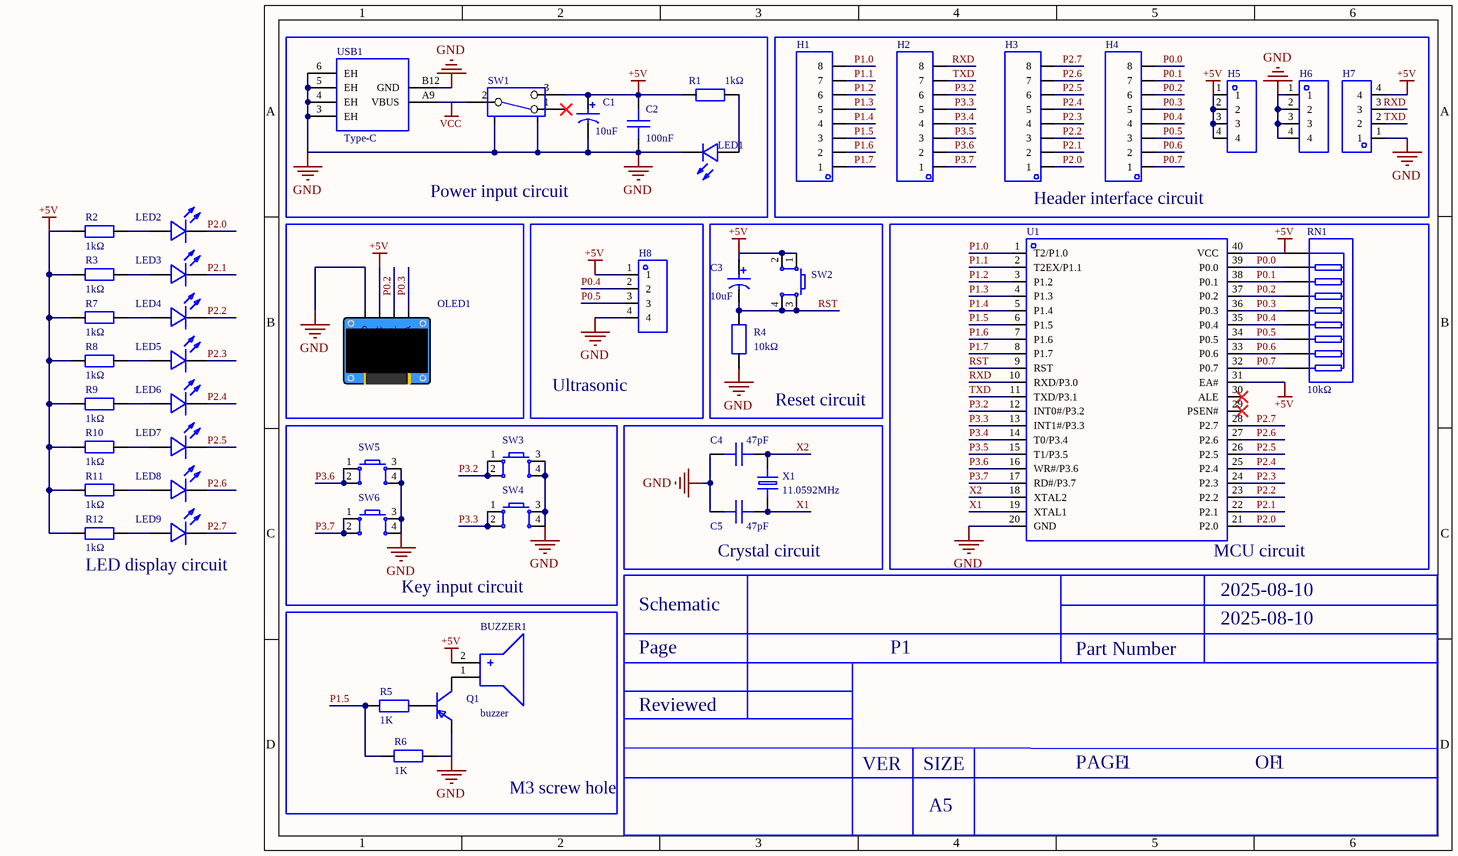
[diagram p0: MISC49889-2.schdoc]
# Altium project MISC49889-3.PrjPcb
1 sheet, 47 parts. Net scope: global (net labels, ports and power ports of the same name join across sheets).
Board file: MISC49889.pcbdoc

## Sheet MISC49889-2.schdoc
size 210 x 149 mm; Version: V1.0; @Project Name: MISC49889; @Page Count: 1; @Update Date: 2025-08-10; @Create Date: 2025-08-10; @Schematic Name: MISC49889; @Page No: 1; @Board Name: MISC49889; @Create Time: 18:24:45; @Update Time: 00:13:02

### Parts
BUZZER1  buzzer  [BUZ-TH_BD12.0-P6.00-D0.9-RD]
C1  10uF  [CAP-TH_BD5.0-P2.00-D0.8-FD]
C2  100nF  [CAP-TH_L8.5-W5.0-P5.00-D1.2]
C3  10uF  [CAP-TH_BD5.0-P2.00-D0.8-FD]
C4  47pF  [CAP-TH_L4.5-W3.0-P5.00-D1.2]
C5  47pF  [CAP-TH_L4.5-W3.0-P5.00-D1.2]
H1  (no value)  [HDR-TH_8P-P2.54-V-M]
H2  (no value)  [HDR-TH_8P-P2.54-V-M]
H3  (no value)  [HDR-TH_8P-P2.54-V-M]
H4  (no value)  [HDR-TH_8P-P2.54-V-M]
H5  (no value)  [HDR-TH_4P-P2.54-V-M]
H6  (no value)  [HDR-TH_4P-P2.54-V-M]
H7  (no value)  [HDR-TH_4P-P2.54-V-M]
H8  (no value)  [HDR-TH_4P-P2.54-V-F]
LED1  204-10SURD/S530-A3-L  [LED-TH_BD3.0-P2.54-FD]  (value not drawn)
LED2  204-10SYGD/S530-E3  [LED-TH_BD3.8-P2.54-FD]  (value not drawn)
LED3  204-10SYGD/S530-E3  [LED-TH_BD3.8-P2.54-FD]  (value not drawn)
LED4  204-10SYGD/S530-E3  [LED-TH_BD3.8-P2.54-FD]  (value not drawn)
LED5  204-10SYGD/S530-E3  [LED-TH_BD3.8-P2.54-FD]  (value not drawn)
LED6  204-10SYGD/S530-E3  [LED-TH_BD3.8-P2.54-FD]  (value not drawn)
LED7  204-10SYGD/S530-E3  [LED-TH_BD3.8-P2.54-FD]  (value not drawn)
LED8  204-10SYGD/S530-E3  [LED-TH_BD3.8-P2.54-FD]  (value not drawn)
LED9  204-10SYGD/S530-E3  [LED-TH_BD3.8-P2.54-FD]  (value not drawn)
OLED1  (no value)  [0.96OLED_4P]
Q1  (no value)  [S8550P_SOT]
R1  1kΩ  [RES-TH_BD2.5-L6.5-P10.50-D0.6]
R2  1kΩ  [RES-TH_BD2.5-L6.5-P10.50-D0.6]
R3  1kΩ  [RES-TH_BD2.5-L6.5-P10.50-D0.6]
R4  10kΩ  [RES-TH_BD2.4-L6.3-P10.30-D0.6]
R5  1K  [R0603]
R6  1K  [R0603]
R7  1kΩ  [RES-TH_BD2.5-L6.5-P10.50-D0.6]
R8  1kΩ  [RES-TH_BD2.5-L6.5-P10.50-D0.6]
R9  1kΩ  [RES-TH_BD2.5-L6.5-P10.50-D0.6]
R10  1kΩ  [RES-TH_BD2.5-L6.5-P10.50-D0.6]
R11  1kΩ  [RES-TH_BD2.5-L6.5-P10.50-D0.6]
R12  1kΩ  [RES-TH_BD2.5-L6.5-P10.50-D0.6]
RN1  10kΩ  [RES-ARRAY-TH_9P-P2.54-D1.0]
SW1  SS-12D02-VG4  [SW-TH_SS-12D02-VG4]  (value not drawn)
SW2  (no value)  [SW-TH_4P-L6.0-W6.0-P4.50-LS6.5]
SW3  (no value)  [SW-TH_4P-L6.0-W6.0-P4.50-LS6.5]
SW4  (no value)  [SW-TH_4P-L6.0-W6.0-P4.50-LS6.5]
SW5  (no value)  [SW-TH_4P-L6.0-W6.0-P4.50-LS6.5]
SW6  (no value)  [SW-TH_4P-L6.0-W6.0-P4.50-LS6.5]
U1  STC89C52RC-40I-PDIP40  [DIP-40_L52.0-W13.7-P2.54-LS15.2-BL]  (value not drawn)
USB1  Connector Type: Type-C  [USB-C-TH_TYPE-C-31-M-33]  (hidden comment: TYPE-C-31-M-33)
X1  11.0592MHz  [HC-49US_L11.5-W4.5-P4.88]

### Blocks framed on the sheet
Power input circuit: C1 C2 LED1 R1 SW1 USB1
Header interface circuit: H1-H7
Ultrasonic: H8
Reset circuit: C3 R4 SW2
MCU circuit: RN1 U1
Key input circuit: SW3-SW6
Crystal circuit: C4 C5 X1
M3 screw hole: BUZZER1 Q1 R5 R6

### Nets
+5V: BUZZER1.2(+) C1.1 C2.2 C3.1 H5.1 H5.2 H5.3 H5.4 H7.4 H8.1 OLED1.2(VCC) R1.1 R2.1 R3.1 R7.1 R8.1 R9.1 R10.1 R11.1 R12.1 RN1.1 SW1.3 SW2.1 SW2.2 U1.31(EA#) U1.40(VCC)
GND: C1.2 C2.1 C4.1 C5.1 H6.1 H6.2 H6.3 H6.4 H7.1 H8.4 LED1.2(K) OLED1.1(GND) Q1.2(E) R4.1 R6.2 SW1.4 SW1.5 SW3.3 SW3.4 SW4.3 SW4.4 SW5.3 SW5.4 SW6.3 SW6.4 U1.20(GND) USB1.3(EH) USB1.4(EH) USB1.5(EH) USB1.6(EH) USB1.B12(GND)
VCC: SW1.2 USB1.A9(VBUS)
P0.0: H4.8 RN1.2 U1.39(P0.0)
P0.1: H4.7 RN1.3 U1.38(P0.1)
P0.2: H4.6 OLED1.3(SCL) RN1.4 U1.37(P0.2)
P0.3: H4.5 OLED1.4(SDA) RN1.5 U1.36(P0.3)
P0.4: H4.4 H8.2 RN1.6 U1.35(P0.4)
P0.5: H4.3 H8.3 RN1.7 U1.34(P0.5)
P0.6: H4.2 RN1.8 U1.33(P0.6)
P0.7: H4.1 RN1.9 U1.32(P0.7)
P1.0: H1.8 U1.1(T2/P1.0)
P1.1: H1.7 U1.2(T2EX/P1.1)
P1.2: H1.6 U1.3(P1.2)
P1.3: H1.5 U1.4(P1.3)
P1.4: H1.4 U1.5(P1.4)
P1.5: H1.3 R5.1 R6.1 U1.6(P1.5)
P1.6: H1.2 U1.7(P1.6)
P1.7: H1.1 U1.8(P1.7)
P2.0: H3.1 LED2.2(K) U1.21(P2.0)
P2.1: H3.2 LED3.2(K) U1.22(P2.1)
P2.2: H3.3 LED4.2(K) U1.23(P2.2)
P2.3: H3.4 LED5.2(K) U1.24(P2.3)
P2.4: H3.5 LED6.2(K) U1.25(P2.4)
P2.5: H3.6 LED7.2(K) U1.26(P2.5)
P2.6: H3.7 LED8.2(K) U1.27(P2.6)
P2.7: H3.8 LED9.2(K) U1.28(P2.7)
P3.2: H2.6 SW3.1 SW3.2 U1.12(INT0#/P3.2)
P3.3: H2.5 SW4.1 SW4.2 U1.13(INT1#/P3.3)
P3.4: H2.4 U1.14(T0/P3.4)
P3.5: H2.3 U1.15(T1/P3.5)
P3.6: H2.2 SW5.1 SW5.2 U1.16(WR#/P3.6)
P3.7: H2.1 SW6.1 SW6.2 U1.17(RD#/P3.7)
RST: C3.2 R4.2 SW2.3 SW2.4 U1.9(RST)
RXD: H2.8 H7.3 U1.10(RXD/P3.0)
TXD: H2.7 H7.2 U1.11(TXD/P3.1)
X1: C5.2 U1.19(XTAL1) X1.1
X2: C4.2 U1.18(XTAL2) X1.2
NetBUZZER1_1: BUZZER1.1(-) Q1.3(C)
NetLED1_1: LED1.1(A) R1.2
NetLED2_1: LED2.1(A) R2.2
NetLED3_1: LED3.1(A) R3.2
NetLED4_1: LED4.1(A) R7.2
NetLED5_1: LED5.1(A) R8.2
NetLED6_1: LED6.1(A) R9.2
NetLED7_1: LED7.1(A) R10.2
NetLED8_1: LED8.1(A) R11.2
NetLED9_1: LED9.1(A) R12.2
NetQ1_1: Q1.1(B) R5.2

Not connected (* = marked no-connect by the designer): SW1 1*; U1 29(PSEN#)* 30(ALE)*

### Notes on the sheet
- LED display circuit
- 2025-08-10
- Schematic
- Page
- P1
- Part Number
- Reviewed
- VER
- A5
- SIZE
- PAGE
- 1
- OF

### Library data of the parts
BUZZER1 = buzzer: AddInBom: yes; ModelId: af17e4151ed84fc2a628230bf2376363; ModelTransform: 472.44,472.176,0,270,0,0,0,0,-196.85; Symbol: BUZZER; Device: buzzer; LCSC Part Name: buzzer; SupplierPart: C9900014030; ManufacturerPart: buzzer; Supplier Footprint: buzzer; JLCPCB Part Class: Extended library; Supplier: LCSC; ConvertToPcb: yes; FootprintName: BUZ-TH_BD12.0-P6.00-D0.9-RD; ModelName: BUZ-TH_BD12.0-P6.00-D0.9-RD
C1 C3 = KM106M050D11RR0VH2FP0: Capacitance: 10uF; Tolerance: ±20%; Rated voltage: 50V; Body diameter: 5mm; Body length: 11mm; Lead pitch: 2mm; Operating life: 1000hrs@105℃;; Manufacturer: CX(承兴); Symbol: 10uF 50V 5*11; AddInBom: yes; ModelId: edeeed87cbc746108d01291548c38636; ModelName: CAP-TH_D5.0×H7.0×P2.0; ModelTransform: 197.091,196.7911,0,0,0,0,0,0,-137.795; Value: 10uF; Device: KM106M050D11RR0VH2FP0; LCSC Part Name: 10uF ±20% 50V; SupplierPart: C43345; ManufacturerPart: KM106M050D11RR0VH2FP0; Supplier Footprint: 插件,D5xL11mm; JLCPCB Part Class: Extended Part; Datasheet: https://example.com/upload/public/pdf/source/20211027/06D6BA3719C264B639DC286D935D03EA.pdf; Supplier: LCSC; ConvertToPcb: yes; FootprintName: CAP-TH_BD5.0-P2.00-D0.8-FD; Rated Voltage: 50V; φD: 5mm; L: 11mm; Lead Spacing: 2mm; Lifetime @ Temp: 1000hrs@105℃
C2 = CT4-0805B104K500F3: Capacitance: 100nF; Tolerance: ±10%; Rated voltage: 50V; Temperature coefficient: X7R;; Manufacturer: FH(风华); AddInBom: yes; ModelId: 5610b656e7164072960d9d2d8c7d4fdf; ModelName: CAP-TH_L4.2-W3.8-H3.8-P5.08; ModelTransform: 222.8342,149.606,0,0,0,0,0,0,-118.11; Value: 100nF; Device: CT4-0805B104K500F3; Symbol: CT4-0805B104K500F3; LCSC Part Name: 100nF ±10% 50V; SupplierPart: C84772; ManufacturerPart: CT4-0805B104K500F3; Supplier Footprint: 插件,P=5.08mm; JLCPCB Part Class: Extended Part; Datasheet: https://example.com/upload/public/pdf/source/20161024/1477288669695.pdf; Supplier: LCSC; ConvertToPcb: yes; FootprintName: CAP-TH_L8.5-W5.0-P5.00-D1.2; Voltage Rated: 50V; Temperature Coefficient: X7R
C4 C5 = CC1H470JC74DCH4B10MN: Capacitance: 47pF; Tolerance: ±5%; Rated voltage: 50V; Temperature coefficient: NP0; Lead pitch: 5.08mm; Body diameter: 4.7mm; Body thickness: 2.2mm;; Manufacturer: Dersonic(德尔创); AddInBom: yes; ModelId: 79770350bfc84ced91525190e1ddc709; ModelName: CAP-TH_BD4.5-W3.0-P5.0; ModelTransform: 222.2505,107.41309,0,0,0,0,0,0,-137.795; Value: 47pF; Device: CC1H470JC74DCH4B10MN; Symbol: CC1H470JC74DCH4B10MN; LCSC Part Name: 47pF ±5% 50V; SupplierPart: C254104; ManufacturerPart: CC1H470JC74DCH4B10MN; Supplier Footprint: 径向引线,P=5.08mm; JLCPCB Part Class: Extended Part; Datasheet: https://example.com/upload/public/pdf/source/20200826/C254104_4D3B00F203A17FA56AC5131CB4177D5E.pdf; Supplier: LCSC; ConvertToPcb: yes; FootprintName: CAP-TH_L4.5-W3.0-P5.00-D1.2; Voltage Rated: 50V; Temperature Coefficient: NP0; Lead Spacing: 5.08mm; φD: 4.7mm; Body Thickness: 2.2mm
H1-H4 = HDR-M_2.54_1x8P: Check: false; Symbol: Header-Male-2.54_1x8; ConvertToPcb: yes; ModelId: f5b96e27511e49e38545e53df2320202; ModelTransform: 807.87244,98.425,0,0,0,0,0,0,-118.11; Device: HDR-M_2.54_1x8P; AddInBom: yes; SupplierPart: C124381; Supplier Footprint: 插件; FootprintName: HDR-TH_8P-P2.54-V-M; ModelName: HDR-TH_8P-P2.54-V-M
H5-H7 = HDR-M_2.54_1x4P: Check: false; Symbol: PZ254V-11-04P; ConvertToPcb: yes; ModelId: 112f4d05e8d64e99ab9a333894bea4f9; ModelName: HDR-TH_4P-P2.54-M-LI-1X4P; ModelTransform: 399.999,104.7242,0,0,0,0,0,0,-118.11; Device: HDR-M_2.54_1x4P; AddInBom: yes; SupplierPart: C492403; Supplier Footprint: 插件; FootprintName: HDR-TH_4P-P2.54-V-M
H8 = HDR-F_2.54_1x4P: Symbol: 2.54-1*4P female; ConvertToPcb: yes; ModelId: d187812051054f85879fcaa51a310d8e; ModelTransform: 419.6842,98.464,0,0,0,0,0,0,-118.11; Device: HDR-F_2.54_1x4P; AddInBom: yes; SupplierPart: C2718488; Supplier Footprint: 插件; FootprintName: HDR-TH_4P-P2.54-V-F; ModelName: HDR-TH_4P-P2.54-V-F
LED1 = 204-10SURD/S530-A3-L: Emitted color: Red; Diode configuration: -; Lens color: Diffused red; Dominant wavelength: 624nm; Peak wavelength: 632nm; Color temperature: -; Test current: 20mA; Power: 60mW; Viewing angle: 40°; Mounting style: -; Operating temperature: -40℃~+85℃;; Manufacturer: EVERLIGHT(亿光); AddInBom: yes; ModelId: a497c992633541038a38947cdc58012f; ModelName: LED-TH-3mm_R; ModelTransform: 141.274,153.327,0,0,0,0,-5.984,0,-137.795; Lamp Holder Type: 3mm round lamp holder; Device: 204-10SURD/S530-A3-L; Symbol: 204-10SURD/S530-A3-L; LCSC Part Name: 红灯 624nm; SupplierPart: C99771; ManufacturerPart: 204-10SURD/S530-A3-L; Supplier Footprint: 插件,D=3mm; JLCPCB Part Class: Extended Part; Datasheet: https://example.com/upload/public/pdf/source/20170504/1493866972127.pdf; Supplier: LCSC; ConvertToPcb: yes; FootprintName: LED-TH_BD3.0-P2.54-FD; Emitted Color: Red; Diode Configuration: -; Lens Color: Diffused red; Dominant Wavelength: 624nm; Peak Wavelength: 632nm; Color Temperature: -; Forward Current: 20mA; Power Dissipation: 60mW; Viewing Angle: 40°; Mounting Sytle: -; Operating Temperature: -40℃~+85℃
LED2-LED9 = 204-10SYGD/S530-E3: Emitted color: Green/Yellow-green;; Manufacturer: EVERLIGHT(亿光); AddInBom: yes; ModelId: 7a5158147ccf41a18926a05cf5a7749d; ModelTransform: 139.516,157.15173,0,0,0,0,-9.054,-1.181,-137.795; Lamp Holder Type: 3mm round lamp holder; Device: 204-10SYGD/S530-E3; Symbol: 204-10SYGD/S530-E3; LCSC Part Name: 普绿/黄绿; SupplierPart: C85161; ManufacturerPart: 204-10SYGD/S530-E3; Supplier Footprint: 插件,D=3mm; JLCPCB Part Class: Extended Part; Datasheet: https://example.com/upload/public/pdf/source/20181205/C85161_54D2881904BBFDED7AAB4D08F0D96F46.pdf; Supplier: LCSC; ConvertToPcb: yes; FootprintName: LED-TH_BD3.8-P2.54-FD; ModelName: LED-TH_BD3.8-P2.54-FD; Emitted Color: Green/Yellow-green
OLED1 = 0.96OLED模块_4P: Device: 0.96OLED module_4P; ConvertToPcb: yes; ModelId: 79c000fdb68d45a296c2e9bedf4f9055; ModelTransform: 1393.69792,1318.895,0,0,0,0,0,-560.079,-137.795; AddInBom: yes; SymbolName: 0.96OLED module_4P; FootprintName: 0.96OLED_4P; Supplier Footprint: 插件; ModelName: 0.96OLED_4P
Q1 = S8550_SOT_PNP: Symbol: PNP; ConvertToPcb: yes; ModelId: 9c0df02d6f3e44e889da37f3e5bf5496; ModelName: SOT-23-3_L2.9-W1.4-P1.90-LS2.5-BR; ModelTransform: 98.43,114.17,37.91,0,0,0,0,0,0; Device: S8550_SOT_PNP; AddInBom: yes; Supplier Footprint: SOT-23; FootprintName: S8550P_SOT
R1-R3 R7-R12 = MFR0W4F1001A50: Resistor type: Metal film resistor; Resistance: 1kΩ; Tolerance: ±1%; Power: 250mW; Temperature coefficient: ±50ppm/℃;; Manufacturer: UNI-ROYAL(厚声); AddInBom: yes; ModelId: 8e6c7ee8323443d1ab8f0504b6353c8c; ModelName: RES-TH_D2.3-L6.5-P10.50; ModelTransform: 431.1015,91.3384,0,0,0,0,0.197,0,-137.795; Value: 1kΩ; Device: MFR0W4F1001A50; Symbol: MFR0W4F1001A50; LCSC Part Name: 金属膜电阻 1kΩ ±1% 250mW; SupplierPart: C57435; ManufacturerPart: MFR0W4F1001A50; Supplier Footprint: 轴向引线; JLCPCB Part Class: Extended Part; Datasheet: https://example.com/upload/public/pdf/source/20170615/1497511028539.pdf; Supplier: LCSC; ConvertToPcb: yes; FootprintName: RES-TH_BD2.5-L6.5-P10.50-D0.6; Type: Metal film resistor; Power(Watts): 250mW; Temperature Coefficient: ±50ppm/℃
R4 = RN1/4W10KFT/BA1: Resistor type: Metal film resistor; Resistance: 10kΩ; Tolerance: ±1%; Power: 250mW; Temperature coefficient: ±50ppm/℃; Max working voltage: 250V; Operating temperature range: -55℃~+125℃;; Manufacturer: Tyohm(幸亚电阻); AddInBom: yes; ModelId: 463263665006444ab7a47bd11b0cf956; ModelTransform: 427.165,94.32816,0,0,0,0,0,0,-196.85; Value: 10kΩ; Device: RN1/4W10KFT/BA1; Symbol: RN 1/4W 10K F T/B A1; LCSC Part Name: 金属膜电阻 10kΩ ±1% 250mW; SupplierPart: C410695; ManufacturerPart: RN1/4W10KFT/BA1; Supplier Footprint: 插件; JLCPCB Part Class: Extended Part; Datasheet: https://example.com/upload/public/pdf/source/20190808/C410695_F4C96186075092C4BC649A77CE7E5B2A.pdf; Supplier: LCSC; ConvertToPcb: yes; FootprintName: RES-TH_BD2.4-L6.3-P10.30-D0.6; ModelName: RES-TH_BD2.4-L6.3-P10.30-D0.6; Type: Metal film resistor; Power(Watts): 250mW; Temperature Coefficient: ±50ppm/℃; Overload Voltage (Max): 250V; Operating Temperature Range: -55℃~+125℃
R5 R6 = Res_0603: ConvertToPcb: yes; SymbolName: Resistor; ModelId: fc143cca1e79419f9cd78b61e9279f08; ModelTransform: 31.8897,63.7794,0,90,0,0,0,0,0; Value: 1K; Device: Res_0603; AddInBom: yes; Supplier Footprint: 0603; FootprintName: R0603; ModelName: R0603
RN1 = A09-103JP: Resistance: 10kΩ; Tolerance: ±5%; Power per element: 125mW; Temperature coefficient: ±100ppm/℃; Resistor count: 8; Pin count: 9;; Manufacturer: FH(风华); AddInBom: yes; ModelId: d106c67f29e14d8080ba548247a719a1; ModelName: SIP-9_L22.8-W3.0-H8.5-P2.54; ModelTransform: 917.49722,118.11,0,0,0,0,0,0,-137.795; Number of Resistors: 8; Value: 10kΩ; Device: A09-103JP; Symbol: A09-103JP; LCSC Part Name: 10kΩ ±5%; SupplierPart: C8692; ManufacturerPart: A09-103JP; Supplier Footprint: SIP-9-2.54mm; JLCPCB Part Class: Extended Part; Datasheet: https://example.com/upload/public/pdf/source/20140224/1457706855244.pdf; Supplier: LCSC; ConvertToPcb: yes; FootprintName: RES-ARRAY-TH_9P-P2.54-D1.0; Power(Watts): 125mW; Temperature Coefficient: ±100ppm/℃; Number of Pins: 9
SW1 = SS-12D02-VG4_C136719: Rated current (DC): -; Rated voltage (DC): -; Rated current (AC): -; Rated voltage (AC): -; Circuit configuration: SPDT; Mounting style: Through-hole; Mechanical life: 5000; Actuator shape: Rectangular post; Pin style: PC pin; Operating temperature: -25℃~+70℃; Switch height: 8.7mm;; Manufacturer: 韩国韩荣; AddInBom: yes; ModelId: 4321fe59a4074cbfb4989553f297c68f; ModelTransform: 334.646,188.683,0,0,0,0,0,0,-137.795; Mechanical Life: 5000; Pin Style: PC pin; Device: SS-12D02-VG4_C136719; Symbol: SS-12D02-VG4; LCSC Part Name: SS-12D02-VG4; SupplierPart: C136719; ManufacturerPart: SS-12D02-VG4; Supplier Footprint: 插件; JLCPCB Part Class: Extended Part; Datasheet: https://example.com/upload/public/pdf/source/20171030/C136719_15093664985151068208.pdf; Supplier: LCSC; ConvertToPcb: yes; FootprintName: SW-TH_SS-12D02-VG4; ModelName: SW-TH_SS-12D02-VG4; Current Rating (DC): -; Voltage Rating (DC): -; Current Rating (AC): -; Voltage Rating (AC): -; Circuit: SPDT; Mounting Sytle: Through-hole; Actuator Style: Rectangular post; Operating Temperature: -25℃~+70℃; Switch Height: 8.7mm
SW2-SW6 = Key_TH_6x6x6: Contact current: 50mA; Rated voltage (DC): 12V; Insulation resistance: 100MΩ; Circuit configuration: SPST; Mounting style: Through-hole; Button shape: Round; Button/cap color: Black; Actuation force: 260gf@±30gf; Operating temperature: -25℃~+70℃; Pin style: PC pin; Switch length: 6mm; Switch width: 6mm; Switch height: 6mm; With bracket: No;; Symbol: Tactile switch; ConvertToPcb: yes; ModelId: 20eee248bc684ccd8cbdbb1d0d91ec6f; ModelName: SW-TH_4P-L6.0-W6.0-H5.0-LS6.5-P4.50; ModelTransform: 236.22,323.03,0,90,0,0,0,0,-137.795; Device: Key_TH_6x6x6; AddInBom: yes; Supplier Footprint: 插件; FootprintName: SW-TH_4P-L6.0-W6.0-P4.50-LS6.5
  SW2: Supplier Part: F
  SW3-SW6: SupplierPart: C2837516
U1 = STC89C52RC-40I-PDIP40: CPU core: 51 series; Max CPU frequency: -; Operating voltage: 3.3V~5.5V; Internal oscillator: -; External clock frequency range: -; Program FLASH size: 8KB; Total RAM: 512Byte; EEPROM/data FLASH size: 4KB; GPIO count: 35; ADC (units/channels/bits): -; DAC (units/channels/bits): -; (E)PWM (units/channels/bits): -; 8-bit Timer count: -; 16-bit Timer count: 3; 32-bit Timer count: -; Internal comparator count: -; U(S)ART count: 1; I2C count: -; I2S count: -;; Manufacturer: STC(宏晶); AddInBom: yes; ModelId: 16d4686a009b4ddca948f91eddb57b14; ModelName: DIP-40_L52.3-W13.8-H4.0-LS15.24-P2.54; ModelTransform: 2059.051,615.743,0,0,0,0,0,0,-118.11; GPIO Ports Number: 35; 16Bit Timer Number: 3; U(S)ART Number: 1; Peripherals / Functions / Protocol Stacks: Watchdog; Manufacturer Part: STC89C52RC-40I-PDIP40; Device: STC89C52RC-40I-PDIP40; Symbol: STC89C52RC-40I; LCSC Part Name: 51系列 闪存：8KB RAM：512Byte; SupplierPart: C14022; Supplier Footprint: DIP-40; JLCPCB Part Class: Extended Part; Datasheet: https://example.com/upload/public/pdf/source/20210104/C14022_3E6032FDBB5DBC6F971AD019A8472F5B.pdf; Supplier: LCSC; ConvertToPcb: yes; FootprintName: DIP-40_L52.0-W13.7-P2.54-LS15.2-BL; CPU Core: 51 series; Maximum Frequency: -; Supply Voltage Range: 3.3V~5.5V; Internal Oscillator: -; External Clock Frequency Rang: -; Program FLASH Size: 8KB; RAM Size: 512Byte; EEPROM/Data FLASH Size: 4KB; ADC (Units/Channels/bits): -; DAC (Units/Channels/bits): -; (E)PWM (Units/Channels/bits): -; 8Bit Timer Number: -; 32Bit Timer Number: -; CMP Number: -; I2C Number: -; I2S Number: -; (Q)SPI Number: -; CAN Number: -; USB (H/D/OTG): -; Operating Temperature Range: -40℃~+85℃
USB1 = TYPE-C-31-M-33: Connector type: Type-C; Standard: -; Gender: Female; Contact count: 2; Port count: 1; Mounting style: Right angle; Rated current - power: 3A; Operating temperature range: -30℃~+80℃;; Manufacturer: 韩国韩荣; AddInBom: yes; ModelId: 27f3aacc3fa94d3fb0646588322915d8; ModelTransform: 351.9678,269.6845,0,0,0,0,0,-45.276,-78.74; Number of Contacts: 2; Number of Ports: 1; Device: TYPE-C-31-M-33; Symbol: TYPE-C-31-M-33; LCSC Part Name: Type-C 母座 弯插; SupplierPart: C2848624; ManufacturerPart: TYPE-C-31-M-33; Supplier Footprint: 插件; JLCPCB Part Class: Extended Part; Datasheet: https://example.com/upload/public/pdf/source/20210810/4286DADA658895E6A7755A4FC585FBE4.pdf; Supplier: LCSC; ConvertToPcb: yes; FootprintName: USB-C-TH_TYPE-C-31-M-33; ModelName: USB-C-TH_TYPE-C-31-M-33; Mounting Style: Right angle; Current Rating - Power (Max): 3A; Operating Temperature Range: -30℃~+80℃
X1 = TAXD11.0592M2GLFBET2T: Crystal type: 49S crystal; Frequency: 11.0592MHz; Frequency tolerance: ±30ppm; Frequency stability: ±30ppm; Load capacitance: 20pF; ESR: 50Ω; Operating temperature: -;; Manufacturer: TAE(雅晶鑫); Symbol: HC-49S11.0592MHZ20PF30PPM; AddInBom: yes; ModelId: a8e34f6c394c4d60ace7720f62d1ccdf; ModelName: HC-49US_L11.0-W4.5-H3.5-P4.88; ModelTransform: 432.46488,177.165,0,0,0,0,0,0,-137.795; Value: 11.0592MHz; Device: TAXD11.0592M2GLFBET2T; LCSC Part Name: 11.0592MHz ±30ppm 20pF; SupplierPart: C127675; ManufacturerPart: TAXD11.0592M2GLFBET2T; Supplier Footprint: HC-49S; JLCPCB Part Class: Extended Part; Datasheet: https://example.com/upload/public/pdf/source/20170914/C127675_1505359414738967689.pdf; Supplier: LCSC; ConvertToPcb: yes; FootprintName: HC-49US_L11.5-W4.5-P4.88; Crystal Type: 49S crystal; Frequency Tolerance: ±30ppm; Frequency Stability: ±30ppm; Load Capacitance: 20pF; Equivalent Series Resistance (ESR): 50Ω; Operating Temperature: -